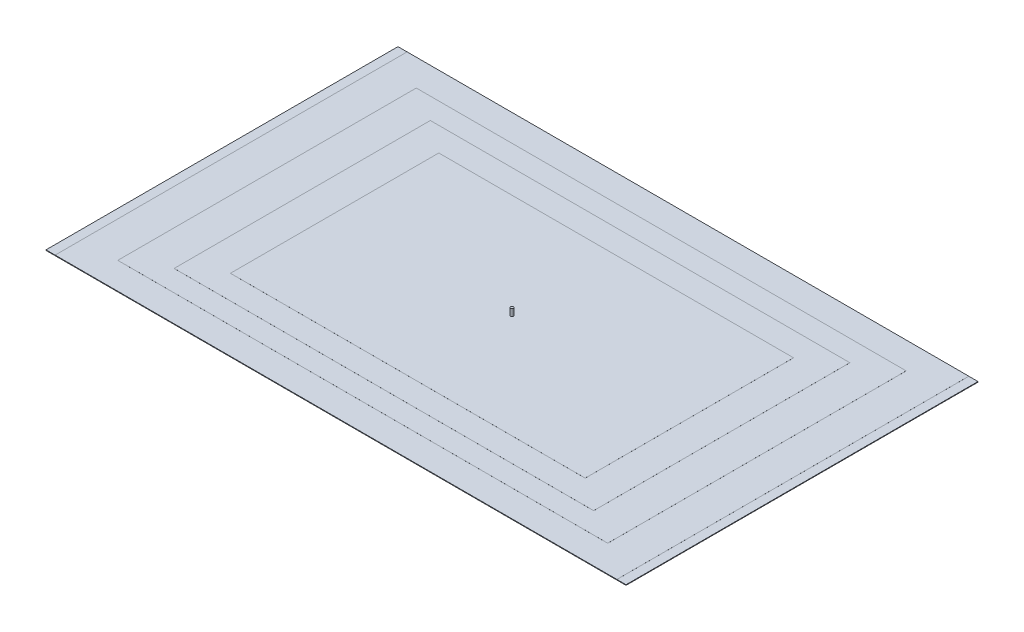
SolidWorks part; units mm, degrees
ref_plane "前基準面" through (0, 0, 0) normal (0, 0, 1) x (1, 0, 0)
ref_plane "上基準面" through (0, 0, 0) normal (0, 1, 0) x (1, 0, 0)
ref_plane "右基準面" through (0, 0, 0) normal (1, 0, 0) x (0, 0, -1)
sketch "草图1" plane through (0, 0, 0) normal (0, 1, 0) x (1, 0, 0)
  line L1 (-1030, -625) -> (1030, -625)
  line L2 (-1030, -625) -> (-1030, 625)
  line L3 (-1030, 625) -> (1030, 625)
  line L4 (1030, -625) -> (1030, 625)
  line L5 (-1030, -625) -> (1030, 625) construction
  line L6 (-1030, 625) -> (1030, -625) construction
  point P0 (0, 0)
  dimension "D1" = 2060
  dimension "D2" = 1250
extrude "凸台-拉伸1" add sketch "草图1" along normal mid plane 2
sketch "草图2" plane through (0, 1, 0) normal (0, 1, 0) x (1, 0, 0)
  line L0 (1030, 625) -> (-1030, 625) construction
  line L1 (-997.5, -625) -> (997.5, -625)
  line L2 (-997.5, -625) -> (-997.5, 625)
  line L3 (-997.5, 625) -> (997.5, 625)
  line L4 (997.5, -625) -> (997.5, 625)
  line L5 (-997.5, -625) -> (997.5, 625) construction
  line L6 (-997.5, 625) -> (997.5, -625) construction
  point P0 (0, 0)
  dimension "D1" = 1995
  dimension "D2" = 1250
extrude "凸台-拉伸2" add sketch "草图2" along normal blind 0.1 separate body
sketch "草图3" plane through (0, 1.1, 0) normal (0, 1, 0) x (1, 0, 0)
  line L1 (-870, -530) -> (870, -530)
  line L2 (-870, -530) -> (-870, 530)
  line L3 (-870, 530) -> (870, 530)
  line L4 (870, -530) -> (870, 530)
  line L5 (-870, -530) -> (870, 530) construction
  line L6 (-870, 530) -> (870, -530) construction
  point P0 (0, 0)
  dimension "D1" = 1740
  dimension "D2" = 1060
extrude "凸台-拉伸5" add sketch "草图3" along normal blind 0.1 separate body
sketch "草图4" plane through (0, 1.2, 0) normal (0, 1, 0) x (1, 0, 0)
  line L1 (-745, -455) -> (745, -455)
  line L2 (-745, -455) -> (-745, 455)
  line L3 (-745, 455) -> (745, 455)
  line L4 (745, -455) -> (745, 455)
  line L5 (-745, -455) -> (745, 455) construction
  line L6 (-745, 455) -> (745, -455) construction
  point P0 (0, 0)
  dimension "D1" = 1490
  dimension "D2" = 910
extrude "凸台-拉伸6" add sketch "草图4" along normal blind 0.1 separate body
sketch "草图5" plane through (0, 1.3, 0) normal (0, 1, 0) x (1, 0, 0)
  line L1 (-630, -370) -> (630, -370)
  line L2 (-630, -370) -> (-630, 370)
  line L3 (-630, 370) -> (630, 370)
  line L4 (630, -370) -> (630, 370)
  line L5 (-630, -370) -> (630, 370) construction
  line L6 (-630, 370) -> (630, -370) construction
  point P0 (0, 0)
  dimension "D1" = 1260
  dimension "D2" = 740
extrude "凸台-拉伸7" add sketch "草图5" along normal blind 0.1 separate body
sketch "草图6" plane through (0, 1.4, 0) normal (0, 1, 0) x (1, 0, 0)
  circle A0 centre (0, 0) radius 5
  dimension "D1" = 10
extrude "凸台-拉伸8" add sketch "草图6" along normal mid plane 50
